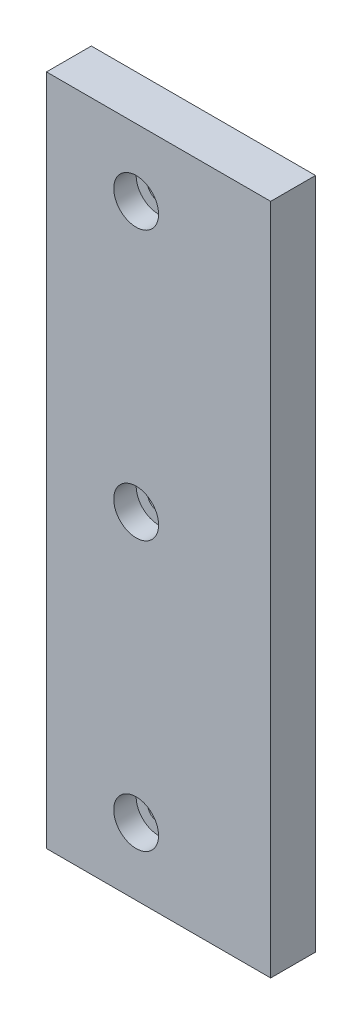
from build123d import *

# Parameters (mm, degrees)
SKETCH1_W           = 50
SKETCH1_H           = 150
BOSS_EXTRUDE1_DEPTH = 5
HOLE1_D             = 5
HOLE1_CBORE_D       = 10
HOLE1_CBORE_DEPTH   = 5


with BuildPart() as part:
    # Sketch1 → Boss-Extrude1 (new, symmetric)
    with BuildSketch(Plane.XY):
        Rectangle(SKETCH1_W, SKETCH1_H)
    extrude(amount=BOSS_EXTRUDE1_DEPTH, both=True)

    # Hole1 (through all)
    with Locations(Plane.XY.offset(5)):
        with Locations((-5, 60), (-5, -60), (-5, 0)):
            CounterBoreHole(HOLE1_D / 2, HOLE1_CBORE_D / 2, HOLE1_CBORE_DEPTH)


solid = part.part
